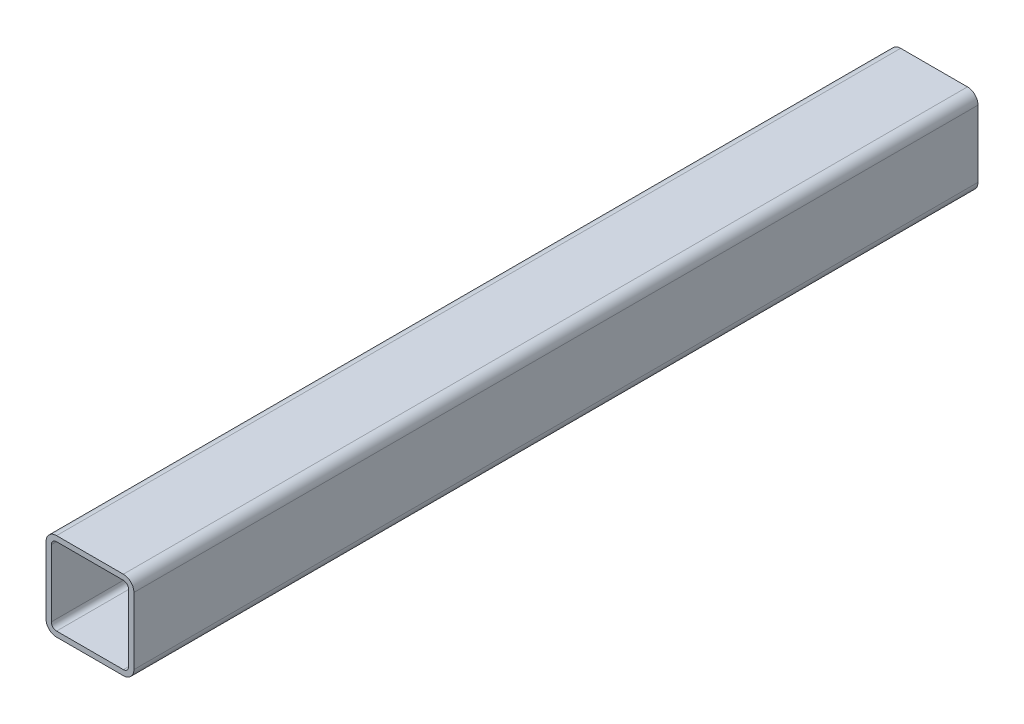
SolidWorks part; units mm, degrees
ref_plane "前视基准面" through (0, 0, 0) normal (0, 0, 1) x (1, 0, 0)
ref_plane "上视基准面" through (0, 0, 0) normal (0, 1, 0) x (1, 0, 0)
ref_plane "右视基准面" through (0, 0, 0) normal (1, 0, 0) x (0, 0, -1)
sketch "草图1" plane through (0, 0, 0) normal (0, 1, 0) x (1, 0, 0)
  line L0 (0, 0) -> (0, 480)
  dimension "D1" = 480
other "Gb／6728-1986方形空心型钢 050 X 50 X 3(1)"
ref_plane "基准面1" through (0, 0, 0) normal (0, 0, -1) x (-1, 0, 0)
sketch "Sketch1" plane through (0, 0, 0) normal (0, 0, -1) x (-1, 0, 0)
  line L0 (-19, -22) -> (19, -22)
  line L1 (-22, -19) -> (-22, 19)
  line L2 (19, 22) -> (-19, 22)
  line L3 (22, 19) -> (22, -19)
  line L4 (-19, -25) -> (19, -25)
  line L5 (-25, -19) -> (-25, 19)
  line L6 (19, 25) -> (-19, 25)
  line L7 (25, 19) -> (25, -19)
  arc A0 (25, 19) -> (19, 25) centre (19, 19) ccw
  arc A1 (19, -25) -> (25, -19) centre (19, -19) ccw
  arc A2 (-25, -19) -> (-19, -25) centre (-19, -19) ccw
  arc A3 (-19, 25) -> (-25, 19) centre (-19, 19) ccw
  arc A4 (-19, 22) -> (-22, 19) centre (-19, 19) ccw
  arc A5 (22, 19) -> (19, 22) centre (19, 19) ccw
  arc A6 (19, -22) -> (22, -19) centre (19, -19) ccw
  arc A7 (-22, -19) -> (-19, -22) centre (-19, -19) ccw
  point P0 (-25, 0)
  point P1 (25, 0)
  point P2 (0, 25)
  point P3 (0, -25)
  point P4 (0, 0)
  point P5 (-25, -25)
  point P6 (25, -25)
  point P7 (25, 25)
  point P8 (-25, 25)
  point P33 (0, 0)
  dimension "D1" = 6
  dimension "Thickness" = 3
  dimension "V_leg" = 50
